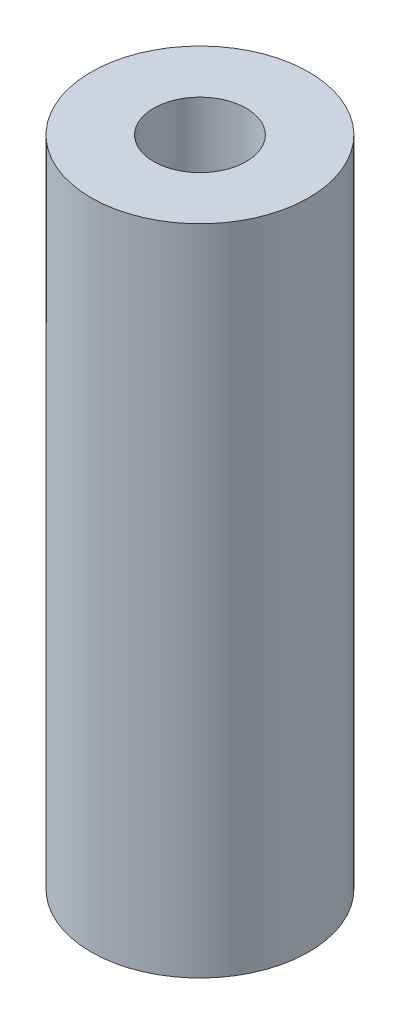
SolidWorks part; units mm, degrees
material "SS400B"
ref_plane "Front Plane" through (0, 0, 0) normal (0, 0, 1) x (1, 0, 0)
ref_plane "Top Plane" through (0, 0, 0) normal (0, 1, 0) x (1, 0, 0)
ref_plane "Right Plane" through (0, 0, 0) normal (1, 0, 0) x (0, 0, -1)
sketch "Sketch1" plane through (0, 0, 0) normal (0, 1, 0) x (1, 0, 0)
  circle A0 centre (0, 0) radius 8
  dimension "D1" = 16
extrude "Boss-Extrude1" add sketch "Sketch1" along normal blind 48
hole_wizard "M8 Tapped Hole1" positions "Sketch2" profile "Sketch3" tap size "M8" standard "GB"
sketch "Sketch2" plane through (0, 48, 0) normal (0, 1, 0) x (1, 0, 0)
  point P0 (0, 0)
sketch "Sketch3" plane through (0, 48, 0) normal (1, 0, 0) x (0, 0, 1)
  line L0 (0, 0) -> (0, 28.0429)
  line L1 (0, 28.0429) -> (3.4, 26)
  line L2 (3.4, 26) -> (3.4, 0)
  line L5 (3.4, 0) -> (0, 0)
  line L10 (0, 28.0429) -> (-3.4, 26) construction
  line L11 (0, -6.35) -> (0, 107.95) construction
  dimension "螺纹孔钻头直径" = 6.8
  dimension "螺纹孔钻头深度" = 26
  dimension "导头角度" = 118
cosmetic thread "Cosmetic Thread1" parameters "D1"=17, "D2"=8
